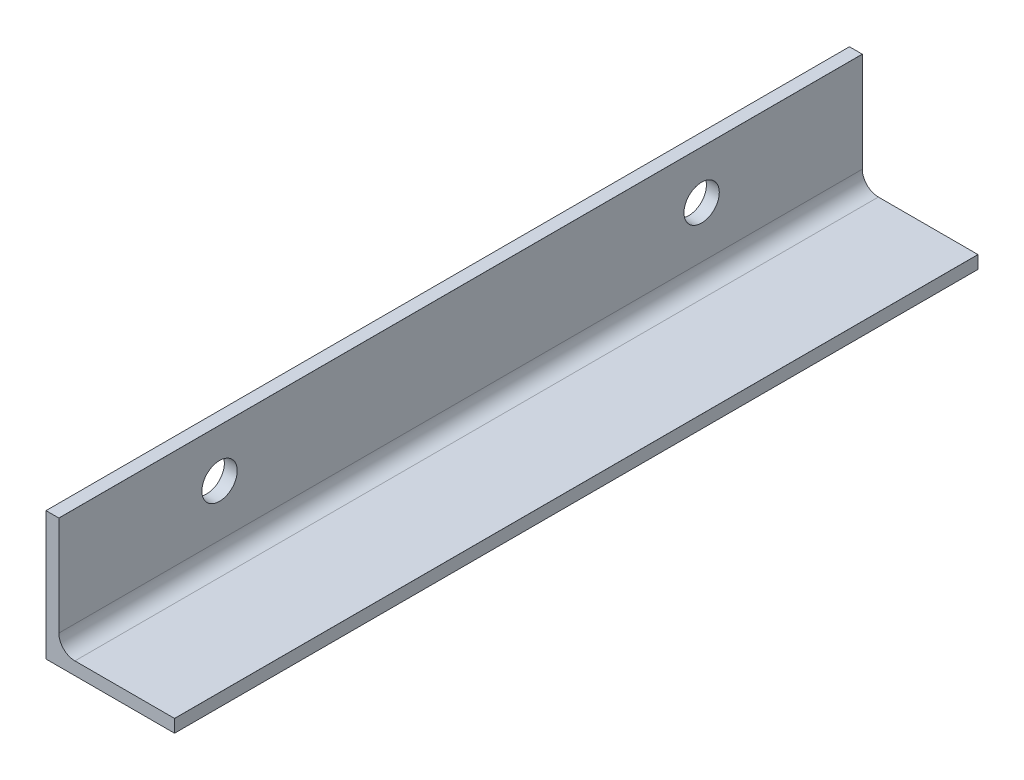
from build123d import *

# Parameters (mm, degrees)
EXTRUDE_1_DEPTH             = 250
HOLE_WIZARD_11_0_11_1_D     = 11
HOLE_WIZARD_11_0_11_1_DEPTH = 10
HOLE_WIZARD_11_0_11_1_TIP   = 3.304733405


with BuildPart() as part:
    # 草图1 → 拉伸1 (new body)
    with BuildSketch(Plane.XY):
        with BuildLine():
            Line((0, 0), (0, 40))
            Line((0, 40), (3.99, 40))
            ThreePointArc((3.99, 40), (3.997071068, 39.997071068), (4, 39.99))
            Line((4, 39.99), (4, 9))
            ThreePointArc((4, 9), (5.464466094, 5.464466094), (9, 4))
            Line((9, 4), (39.99, 4))
            ThreePointArc((39.99, 4), (39.997071068, 3.997071068), (40, 3.99))
            Line((40, 3.99), (40, 0))
            Line((40, 0), (0, 0))
        make_face()
    extrude(amount=EXTRUDE_1_DEPTH)

    # Ø11.0 (11) 直径孔1
    with Locations(Plane.ZY):
        with Locations((200, 25), (50, 25)):
            Hole(HOLE_WIZARD_11_0_11_1_D / 2, depth=HOLE_WIZARD_11_0_11_1_DEPTH)
            with Locations((0, 0, -(HOLE_WIZARD_11_0_11_1_DEPTH + HOLE_WIZARD_11_0_11_1_TIP / 2))):  # 118° drill point
                Cone(0, HOLE_WIZARD_11_0_11_1_D / 2, HOLE_WIZARD_11_0_11_1_TIP, mode=Mode.SUBTRACT)


solid = part.part
